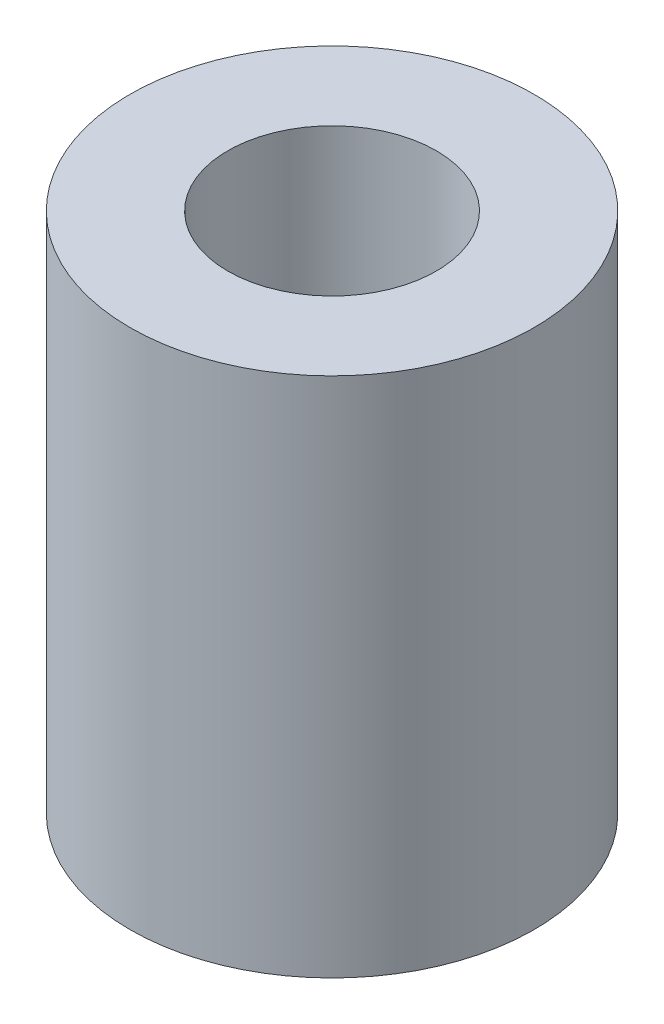
from build123d import *

# Parameters (mm, degrees)
SKETCH_1_R      = 3.1
SKETCH_1_R_2    = 1.6
EXTRUDE_1_DEPTH = 8


with BuildPart() as part:
    # 草图1 → 凸台-拉伸1 (new body)
    with BuildSketch(Plane(origin=(0, 0, 0), x_dir=(1, 0, 0), z_dir=(0, 1, 0))):
        with Locations(Location((0, 0, 0), (0, 0, 270))):
            Circle(SKETCH_1_R)
        with Locations(Location((0, 0, 0), (0, 0, 270))):
            Circle(SKETCH_1_R_2, mode=Mode.SUBTRACT)
    extrude(amount=EXTRUDE_1_DEPTH)


solid = part.part
